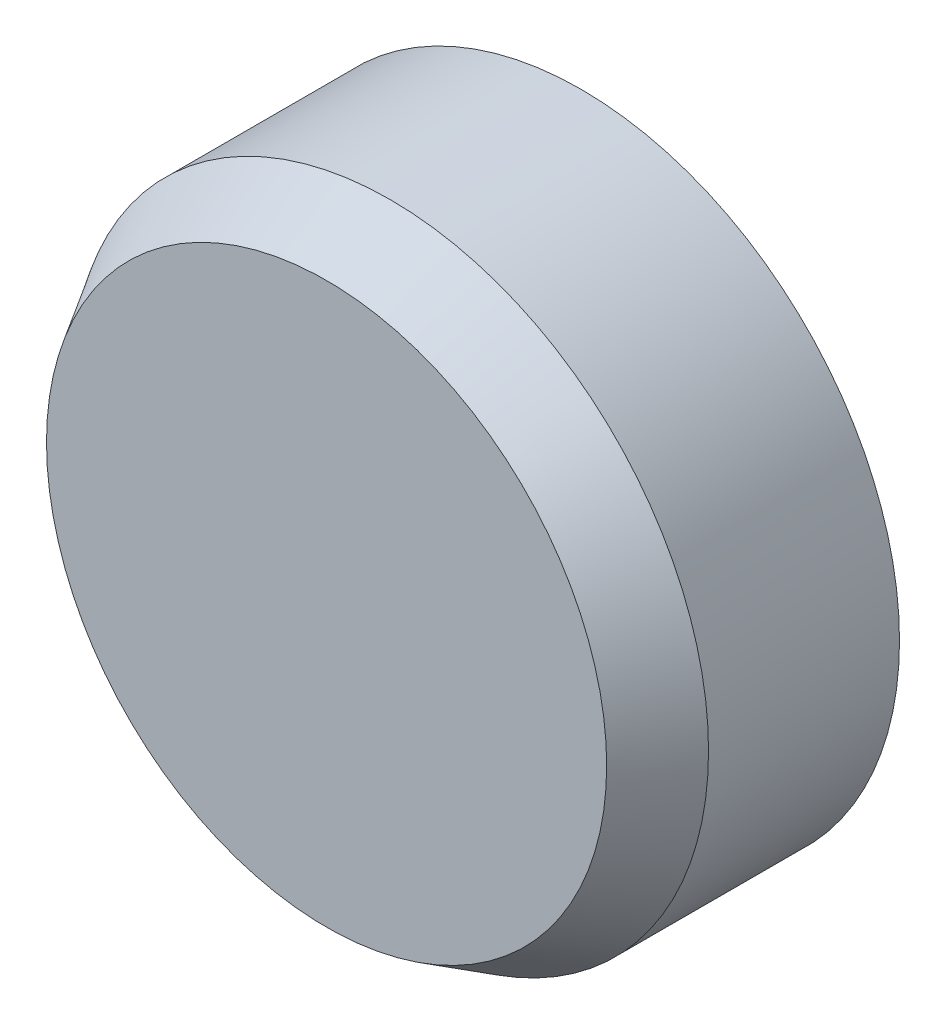
SolidWorks part; units mm, degrees
material "S45C"
ref_plane "Front Plane" through (0, 0, 0) normal (0, 0, 1) x (1, 0, 0)
ref_plane "Top Plane" through (0, 0, 0) normal (0, 1, 0) x (1, 0, 0)
ref_plane "Right Plane" through (0, 0, 0) normal (1, 0, 0) x (0, 0, -1)
sketch "Sketch1" plane through (0, 0, 0) normal (0, 0, 1) x (1, 0, 0)
  circle A0 centre (0, 0) radius 50
  dimension "D1" = 100
extrude "Boss-Extrude1" add sketch "Sketch1" along normal blind 40
chamfer "Chamfer1" distance 10 distance2 6 1 edges at (50, 0, 40)
hole_wizard "M6 Tapped Hole1" positions "Sketch4" profile "Sketch3" tap size "M6" standard "GB"
sketch "Sketch4" plane through (0, 0, 0) normal (0, 0, -1) x (-1, 0, 0)
  point P0 (0, 0)
sketch "Sketch3" plane through (0, 0, 0) normal (1, 0, 0) x (0, 1, 0)
  line L0 (0, 0) -> (0, 18.5022)
  line L1 (0, 18.5022) -> (2.5, 17)
  line L2 (2.5, 17) -> (2.5, 0)
  line L5 (2.5, 0) -> (0, 0)
  line L10 (0, 18.5022) -> (-2.5, 17) construction
  line L11 (0, -6.35) -> (0, 107.95) construction
  dimension "螺纹孔钻头直径" = 5
  dimension "螺纹孔钻头深度" = 17
  dimension "导头角度" = 118
cosmetic thread "Hole thread1" parameters "D1"=12, "D2"=6
